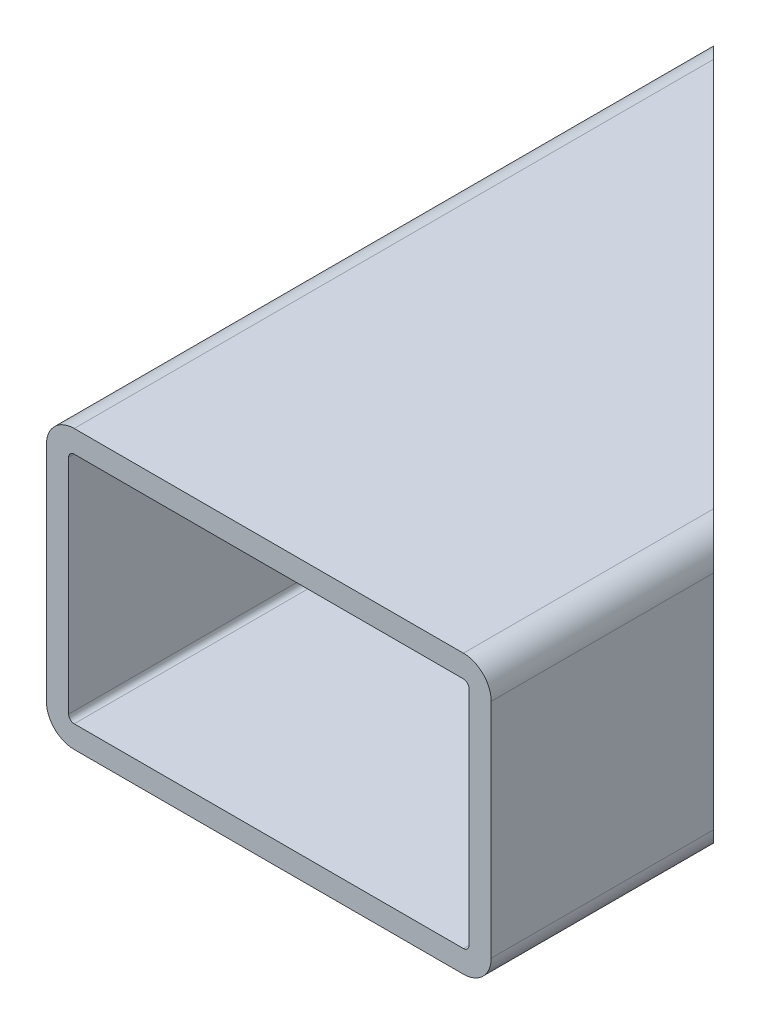
SolidWorks part; units mm, degrees
material "1023 Carbon Steel Plate (SS)"
ref_plane "Front Plane" through (0, 0, 0) normal (0, 0, 1) x (1, 0, 0)
ref_plane "Top Plane" through (0, 0, 0) normal (0, 1, 0) x (1, 0, 0)
ref_plane "Right Plane" through (0, 0, 0) normal (1, 0, 0) x (0, 0, -1)
sketch "Sketch1" plane through (0, 0, 0) normal (0, 0, 1) x (1, 0, 0)
  line L1 (35, 25) -> (-35, 25)
  line L2 (40, 20) -> (40, -20)
  line L3 (35, -25) -> (-35, -25)
  line L4 (-40, 20) -> (-40, -20)
  line L5 (40, 25) -> (-40, -25) construction
  line L6 (40, -25) -> (-40, 25) construction
  arc A0 (-35, -25) -> (-40, -20) centre (-35, -20) cw
  arc A1 (40, -20) -> (35, -25) centre (35, -20) cw
  arc A2 (35, 25) -> (40, 20) centre (35, 20) cw
  arc A3 (-35, 25) -> (-40, 20) centre (-35, 20) ccw
  point P0 (0, 0)
  dimension "D3" = 5
  dimension "D1" = 80
  dimension "D2" = 50
extrude "Boss-Extrude1" add sketch "Sketch1" along normal blind 2200 contours L4 A0 L3 A1 L2 A2 L1 A3
shell "Shell1" thickness 4
sketch "Sketch2" plane through (0, 25, 0) normal (0, 1, 0) x (1, 0, 0)
  line L1 (-25, -849) -> (25, -849) construction
  line L2 (-25, -849) -> (-25, -919) construction
  line L3 (-25, -919) -> (25, -919) construction
  line L4 (25, -849) -> (25, -919) construction
  line L5 (-25, -849) -> (25, -919) construction
  line L6 (-25, -919) -> (25, -849) construction
  line L7 (-25, -1281) -> (25, -1281) construction
  line L8 (-25, -1281) -> (-25, -1351) construction
  line L9 (-25, -1351) -> (25, -1351) construction
  line L10 (25, -1281) -> (25, -1351) construction
  line L11 (-25, -1281) -> (25, -1351) construction
  line L12 (-25, -1351) -> (25, -1281) construction
  line L13 (-35, -2200) -> (-35, 0) construction
  circle A0 centre (-25, -919) radius 3.25
  circle A1 centre (25, -919) radius 3.25
  circle A2 centre (-25, -849) radius 3.25
  circle A3 centre (25, -849) radius 3.25
  circle A4 centre (-25, -1281) radius 3.25
  circle A5 centre (25, -1281) radius 3.25
  circle A6 centre (-25, -1351) radius 3.25
  circle A7 centre (25, -1351) radius 3.25
  point P0 (0, -884)
  point P5 (0, -1316)
  point P14 (-35, -1100)
  dimension "D7" = 6.5
  dimension "D1" = 70
  dimension "D2" = 50
  dimension "D3" = 50
  dimension "D4" = 70
  dimension "D5" = 362
  dimension "D6" = 181
extrude "Cut-Extrude1" cut sketch "Sketch2" against normal blind 10
sketch "Sketch3" plane through (0, -25, 0) normal (0, -1, 0) x (1, 0, 0)
  line L0 (-40, 2200) -> (40, 2120)
  line L1 (40, 2200) -> (40, 0) construction
  line L2 (40, 2120) -> (40, 2200)
  line L3 (40, 2200) -> (-40, 2200)
  line L4 (-35, 1100) -> (784.0884, 1100) construction
  line L5 (-35, 2200) -> (-35, 0) construction
  line L6 (-40, 2200) -> (-40, 0) construction
  line L7 (40, 80) -> (40, 0)
  line L8 (-40, 0) -> (40, 80)
  line L9 (40, 0) -> (-40, 0)
  dimension "D1" = 45
extrude "Cut-Extrude2" cut sketch "Sketch3" against normal blind 2000
sketch "Sketch4" plane through (0, -25, 0) normal (0, -1, 0) x (1, 0, 0)
  line L1 (1017.7021, 2263.36) -> (-1017.7021, 2263.36)
  line L2 (1017.7021, 2263.36) -> (1017.7021, 120)
  line L3 (1017.7021, 120) -> (-1017.7021, 120)
  line L4 (-1017.7021, 2263.36) -> (-1017.7021, 120)
  line L5 (1017.7021, 2263.36) -> (-1017.7021, 120) construction
  line L6 (1017.7021, 120) -> (-1017.7021, 2263.36) construction
  point P0 (0, 1191.68)
  dimension "D1" = 120
extrude "Cut-Extrude3" cut sketch "Sketch4" against normal blind 2000
